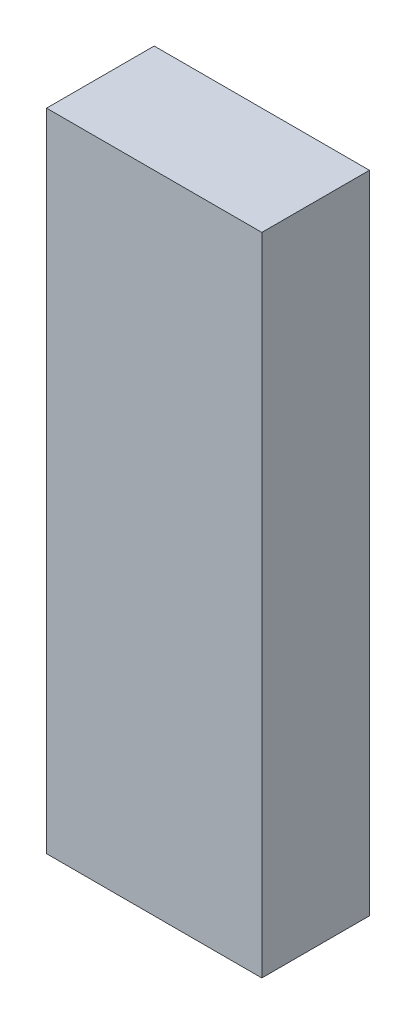
SolidWorks part; units mm, degrees
ref_plane "前视基准面" through (0, 0, 0) normal (0, 0, 1) x (1, 0, 0)
ref_plane "上视基准面" through (0, 0, 0) normal (0, 1, 0) x (1, 0, 0)
ref_plane "右视基准面" through (0, 0, 0) normal (1, 0, 0) x (0, 0, -1)
sketch "草图1" plane through (0, 0, 0) normal (0, 0, 1) x (1, 0, 0)
  line L0 (0, 0) -> (0, 60)
  line L1 (0, 60) -> (150, 60)
  line L2 (150, 60) -> (150, 0)
  line L3 (150, 0) -> (0, 0)
extrude "凸台-拉伸1" add sketch "草图1" along normal blind 10
sketch "草图2" plane through (150, 0, 0) normal (1, 0, 0) x (0, 0, -1)
  line L8 (10, -10) -> (10, 70)
  line L9 (10, 70) -> (-20, 70)
  line L10 (-20, 70) -> (-20, -10)
  line L11 (-20, -10) -> (10, -10)
  line L12 (10, -10) -> (10, 70)
  line L13 (10, 70) -> (-20, 70)
  line L14 (-20, 70) -> (-20, -10)
  line L15 (-20, -10) -> (10, -10)
  dimension "D1" = 10
extrude "切除-拉伸1" cut sketch "草图2" against normal blind 80
sketch "草图3" plane through (0, 0, 10) normal (0, 0, 1) x (1, 0, 0)
  line L0 (0, 60) -> (20, 60)
  line L2 (70, 60) -> (0, 60) construction
  line L4 (20, 60) -> (20, 0)
  line L5 (0, 0) -> (70, 0) construction
  line L6 (20, 0) -> (0, 0)
  line L7 (0, 0) -> (0, 60)
  line L8 (20, 60) -> (70, 60)
  line L9 (70, 60) -> (70, 0)
  line L10 (70, 0) -> (20, 0)
  line M1 (70, 0) -> (70, 60)
  line M2 (70, 60) -> (0, 60)
  line M4 (0, 0) -> (70, 0)
extrude "切除-拉伸3" cut sketch "草图3" against normal blind 10 contours L4 M2 M4 M1
